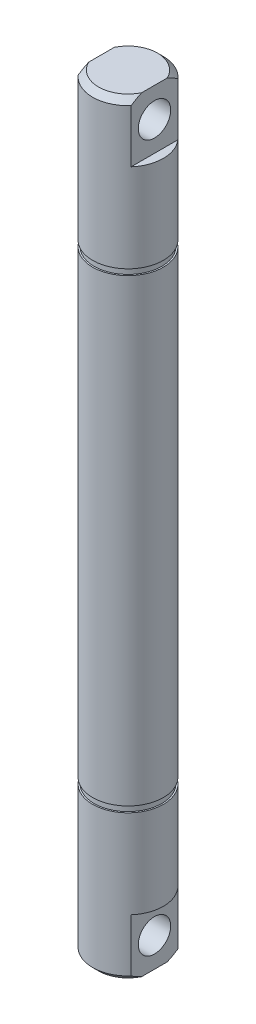
SolidWorks part; units mm, degrees
ref_plane "Front Plane" through (0, 0, 0) normal (0, 0, 1) x (1, 0, 0)
ref_plane "Top Plane" through (0, 0, 0) normal (0, 1, 0) x (1, 0, 0)
ref_plane "Right Plane" through (0, 0, 0) normal (1, 0, 0) x (0, 0, -1)
other "Configuration Table"
sketch "Sketch1" plane through (0, 0, 0) normal (0, 1, 0) x (1, 0, 0)
  circle A0 centre (0, 0) radius 6
  dimension "D1" = 12
extrude "Boss-Extrude1" add sketch "Sketch1" along normal blind 130
sketch "Sketch3" plane through (0, 0, 0) normal (1, 0, 0) x (0, 0, -1)
  line L0 (0, 130) -> (0, 0) construction
  line L1 (6, 130) -> (-6, 130) construction
  line L2 (-6, 0) -> (6, 0) construction
  circle A0 centre (0, 125) radius 2.75
  circle A1 centre (0, 5) radius 2.75
  dimension "D1" = 5.5
  dimension "D3" = 5.5
  dimension "D2" = 5
  dimension "D4" = 5
extrude "Cut-Extrude1" cut sketch "Sketch3" against normal through all both and the other way through all
chamfer "Chamfer1" distance 1 angle 45 2 edges at (0, 0, 6) (0, 130, 6)
ref_plane "Plane1" through (6, 0, 0) normal (1, 0, 0) x (0, 0, -1)
sketch "Sketch5" plane through (6, 0, 0) normal (1, 0, 0) x (0, 0, -1)
  line L1 (-5, -10) -> (5, -10)
  line L2 (-5, -10) -> (-5, 10)
  line L3 (-5, 10) -> (5, 10)
  line L4 (5, -10) -> (5, 10)
  line L5 (-5, -10) -> (5, 10) construction
  line L6 (-5, 10) -> (5, -10) construction
  point P0 (0, 0)
  dimension "D1" = 10
  dimension "D2" = 20
extrude "Cut-Extrude2" cut sketch "Sketch5" against normal blind 1.5
ref_plane "Plane2" through (0, 65, 0) normal (0, -1, 0) x (-1, 0, 0)
mirror "Mirror1" about plane through (0, 0, 0) normal (1, 0, 0) of "Cut-Extrude2"
mirror "Mirror2" about plane through (0, 65, 0) normal (0, -1, 0) of "Mirror1", "Cut-Extrude2"
ref_plane "Plane3" through (0, 155, 0) normal (0, 1, 0) x (1, 0, 0)
ref_plane "Plane4" through (0, 104, 0) normal (0, 1, 0) x (1, 0, 0)
sketch "Sketch7" plane through (0, 104, 0) normal (0, 1, 0) x (1, 0, 0)
  circle A0 centre (0, 0) radius 5.75
  circle A1 centre (0, 0) radius 6
  dimension "D1" = 11.5
extrude "Cut-Extrude3" cut sketch "Sketch7" along normal blind 1
mirror "Mirror3" about plane through (0, 65, 0) normal (0, -1, 0) of "Cut-Extrude3"
